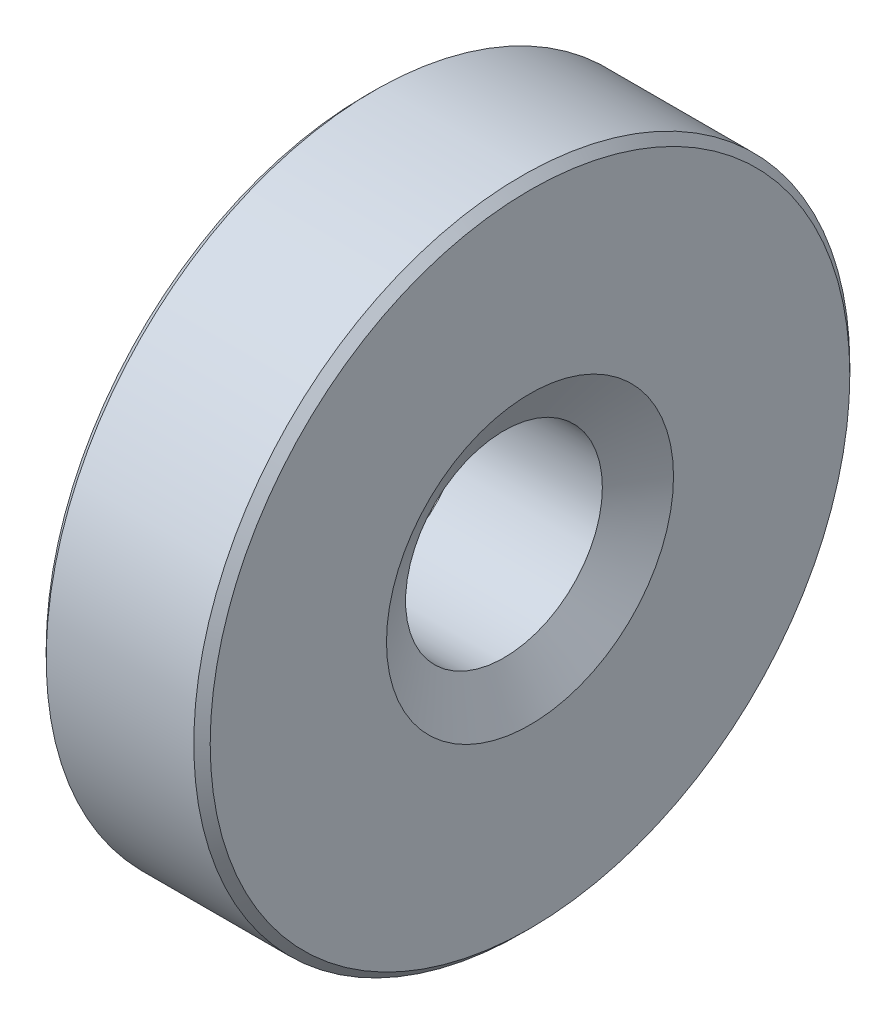
SolidWorks part; units mm, degrees
material "Plain Carbon Steel"
ref_plane "Front Plane" through (0, 0, 0) normal (0, 0, 1) x (1, 0, 0)
ref_plane "Top Plane" through (0, 0, 0) normal (0, 1, 0) x (1, 0, 0)
ref_plane "Right Plane" through (0, 0, 0) normal (1, 0, 0) x (0, 0, -1)
sketch "Sketch1" plane through (0, 0, 0) normal (1, 0, 0) x (0, 0, -1)
  circle A0 centre (0, 0) radius 40
  dimension "D1" = 80
extrude "Extrude1" add sketch "Sketch1" along normal blind 20
sketch "Sketch2" plane through (20, 0, 0) normal (1, 0, 0) x (0, 0, -1)
  circle A0 centre (0, 0) radius 12
  dimension "D1" = 24
extrude "Cut-Extrude1" cut sketch "Sketch2" against normal through all
chamfer "Chamfer1" distance 1 angle 45 2 edges at (0, 0, -40) (20, 0, -40)
chamfer "Chamfer2" distance 5.5 angle 30 1 edges at (20, 0, -12)
